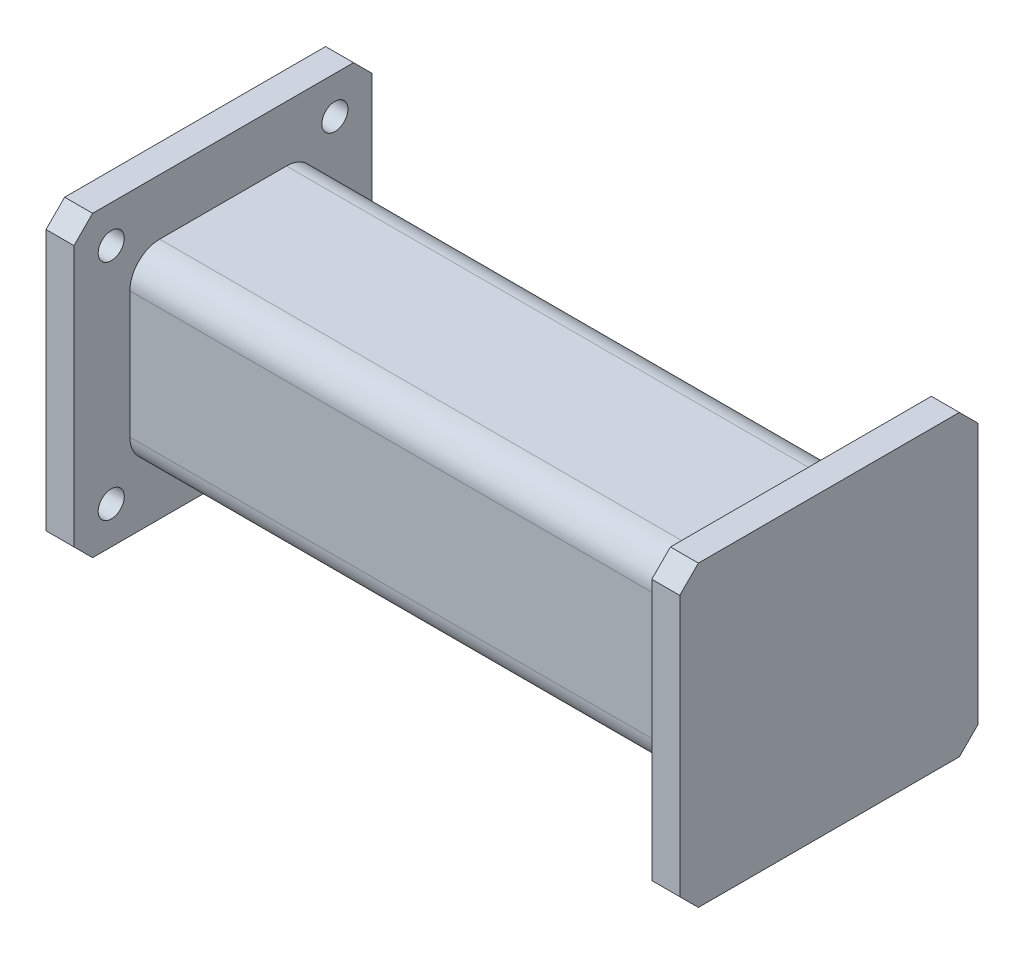
SolidWorks part; units mm, degrees
ref_plane "Front Plane" through (0, 0, 0) normal (0, 0, 1) x (1, 0, 0)
ref_plane "Top Plane" through (0, 0, 0) normal (0, 1, 0) x (1, 0, 0)
ref_plane "Right Plane" through (0, 0, 0) normal (1, 0, 0) x (0, 0, -1)
sketch "Sketch1" plane through (0, 0, 0) normal (1, 0, 0) x (0, 0, -1)
  line L0 (0, 150) -> (10, 160)
  line L1 (10, 0) -> (150, 0)
  line L2 (0, 10) -> (0, 150)
  line L3 (10, 160) -> (150, 160)
  line L4 (160, 10) -> (160, 150)
  line L5 (10, 0) -> (0, 10)
  line L6 (150, 0) -> (160, 10)
  line L7 (160, 150) -> (150, 160)
  point P0 (0, 0)
  point P1 (160, 160)
  point P2 (0, 160)
  point P3 (160, 0)
  dimension "D1" = 160
extrude "Boss-Extrude1" add sketch "Sketch1" along normal blind 15
sketch "Sketch2" plane through (15, 0, 0) normal (1, 0, 0) x (0, 0, -1)
  line L0 (80, 130) -> (80, 5.1672) construction
  line L1 (46, 130) -> (114, 130)
  line L2 (30, 114) -> (30, 46)
  line L3 (46, 30) -> (114, 30)
  line L4 (130, 114) -> (130, 46)
  line L5 (0, 150) -> (0, 10) construction
  line L6 (150, 160) -> (10, 160) construction
  line L7 (46, 122) -> (114, 122)
  line L8 (122, 114) -> (122, 46)
  line L9 (46, 38) -> (114, 38)
  line L10 (38, 114) -> (38, 46)
  arc A0 (114, 130) -> (130, 114) centre (114, 114) cw
  arc A1 (130, 46) -> (114, 30) centre (114, 46) cw
  arc A2 (46, 30) -> (30, 46) centre (46, 46) cw
  arc A3 (30, 114) -> (46, 130) centre (46, 114) cw
  arc A4 (114, 122) -> (122, 114) centre (114, 114) cw
  arc A5 (122, 46) -> (114, 38) centre (114, 46) cw
  arc A6 (46, 38) -> (38, 46) centre (46, 46) cw
  arc A7 (38, 114) -> (46, 122) centre (46, 114) cw
  dimension "D4" = 16
  dimension "D1" = 50
  dimension "D2" = 80
  dimension "D3" = 30
  dimension "D5" = 8
extrude "Boss-Extrude2" add sketch "Sketch2" along normal blind 310
ref_plane "Plane1" through (170, 0, 0) normal (1, 0, 0) x (0, 0, -1)
mirror "Mirror1" about plane through (170, 0, 0) normal (1, 0, 0) of "Boss-Extrude1"
hole_wizard "Ø14.0 (14) Diameter Hole1" positions "3DSketch2" profile "Sketch4" hole size "Ø14.0" standard "ISO"
sketch3d "3DSketch2"
  line L0 (15, 10, -160) -> (15, 150, -160) construction
  line L1 (15, 160, -150) -> (15, 160, -10) construction
  line L2 (15, 150, 0) -> (15, 10, 0) construction
  line L3 (15, 0, -10) -> (15, 0, -150) construction
  point P0 (15, 140, -140)
  point P2 (15, 20, -140)
  point P4 (15, 140, -20)
  point P6 (15, 20, -20)
  dimension "D1" = 20
  dimension "D2" = 20
  dimension "D3" = 20
  dimension "D4" = 20
sketch "Sketch4" plane through (15, 140, -140) normal (0, 1, 0) x (0, 0, -1)
  line L0 (0, 0) -> (0, 15)
  line L1 (0, 15) -> (7, 15)
  line L2 (7, 15) -> (7, 0)
  line L5 (7, 0) -> (0, 0)
  line L11 (0, -6.35) -> (0, 107.95) construction
  dimension "Thru Hole Dia." = 14
  dimension "Thru Hole Depth" = 15
